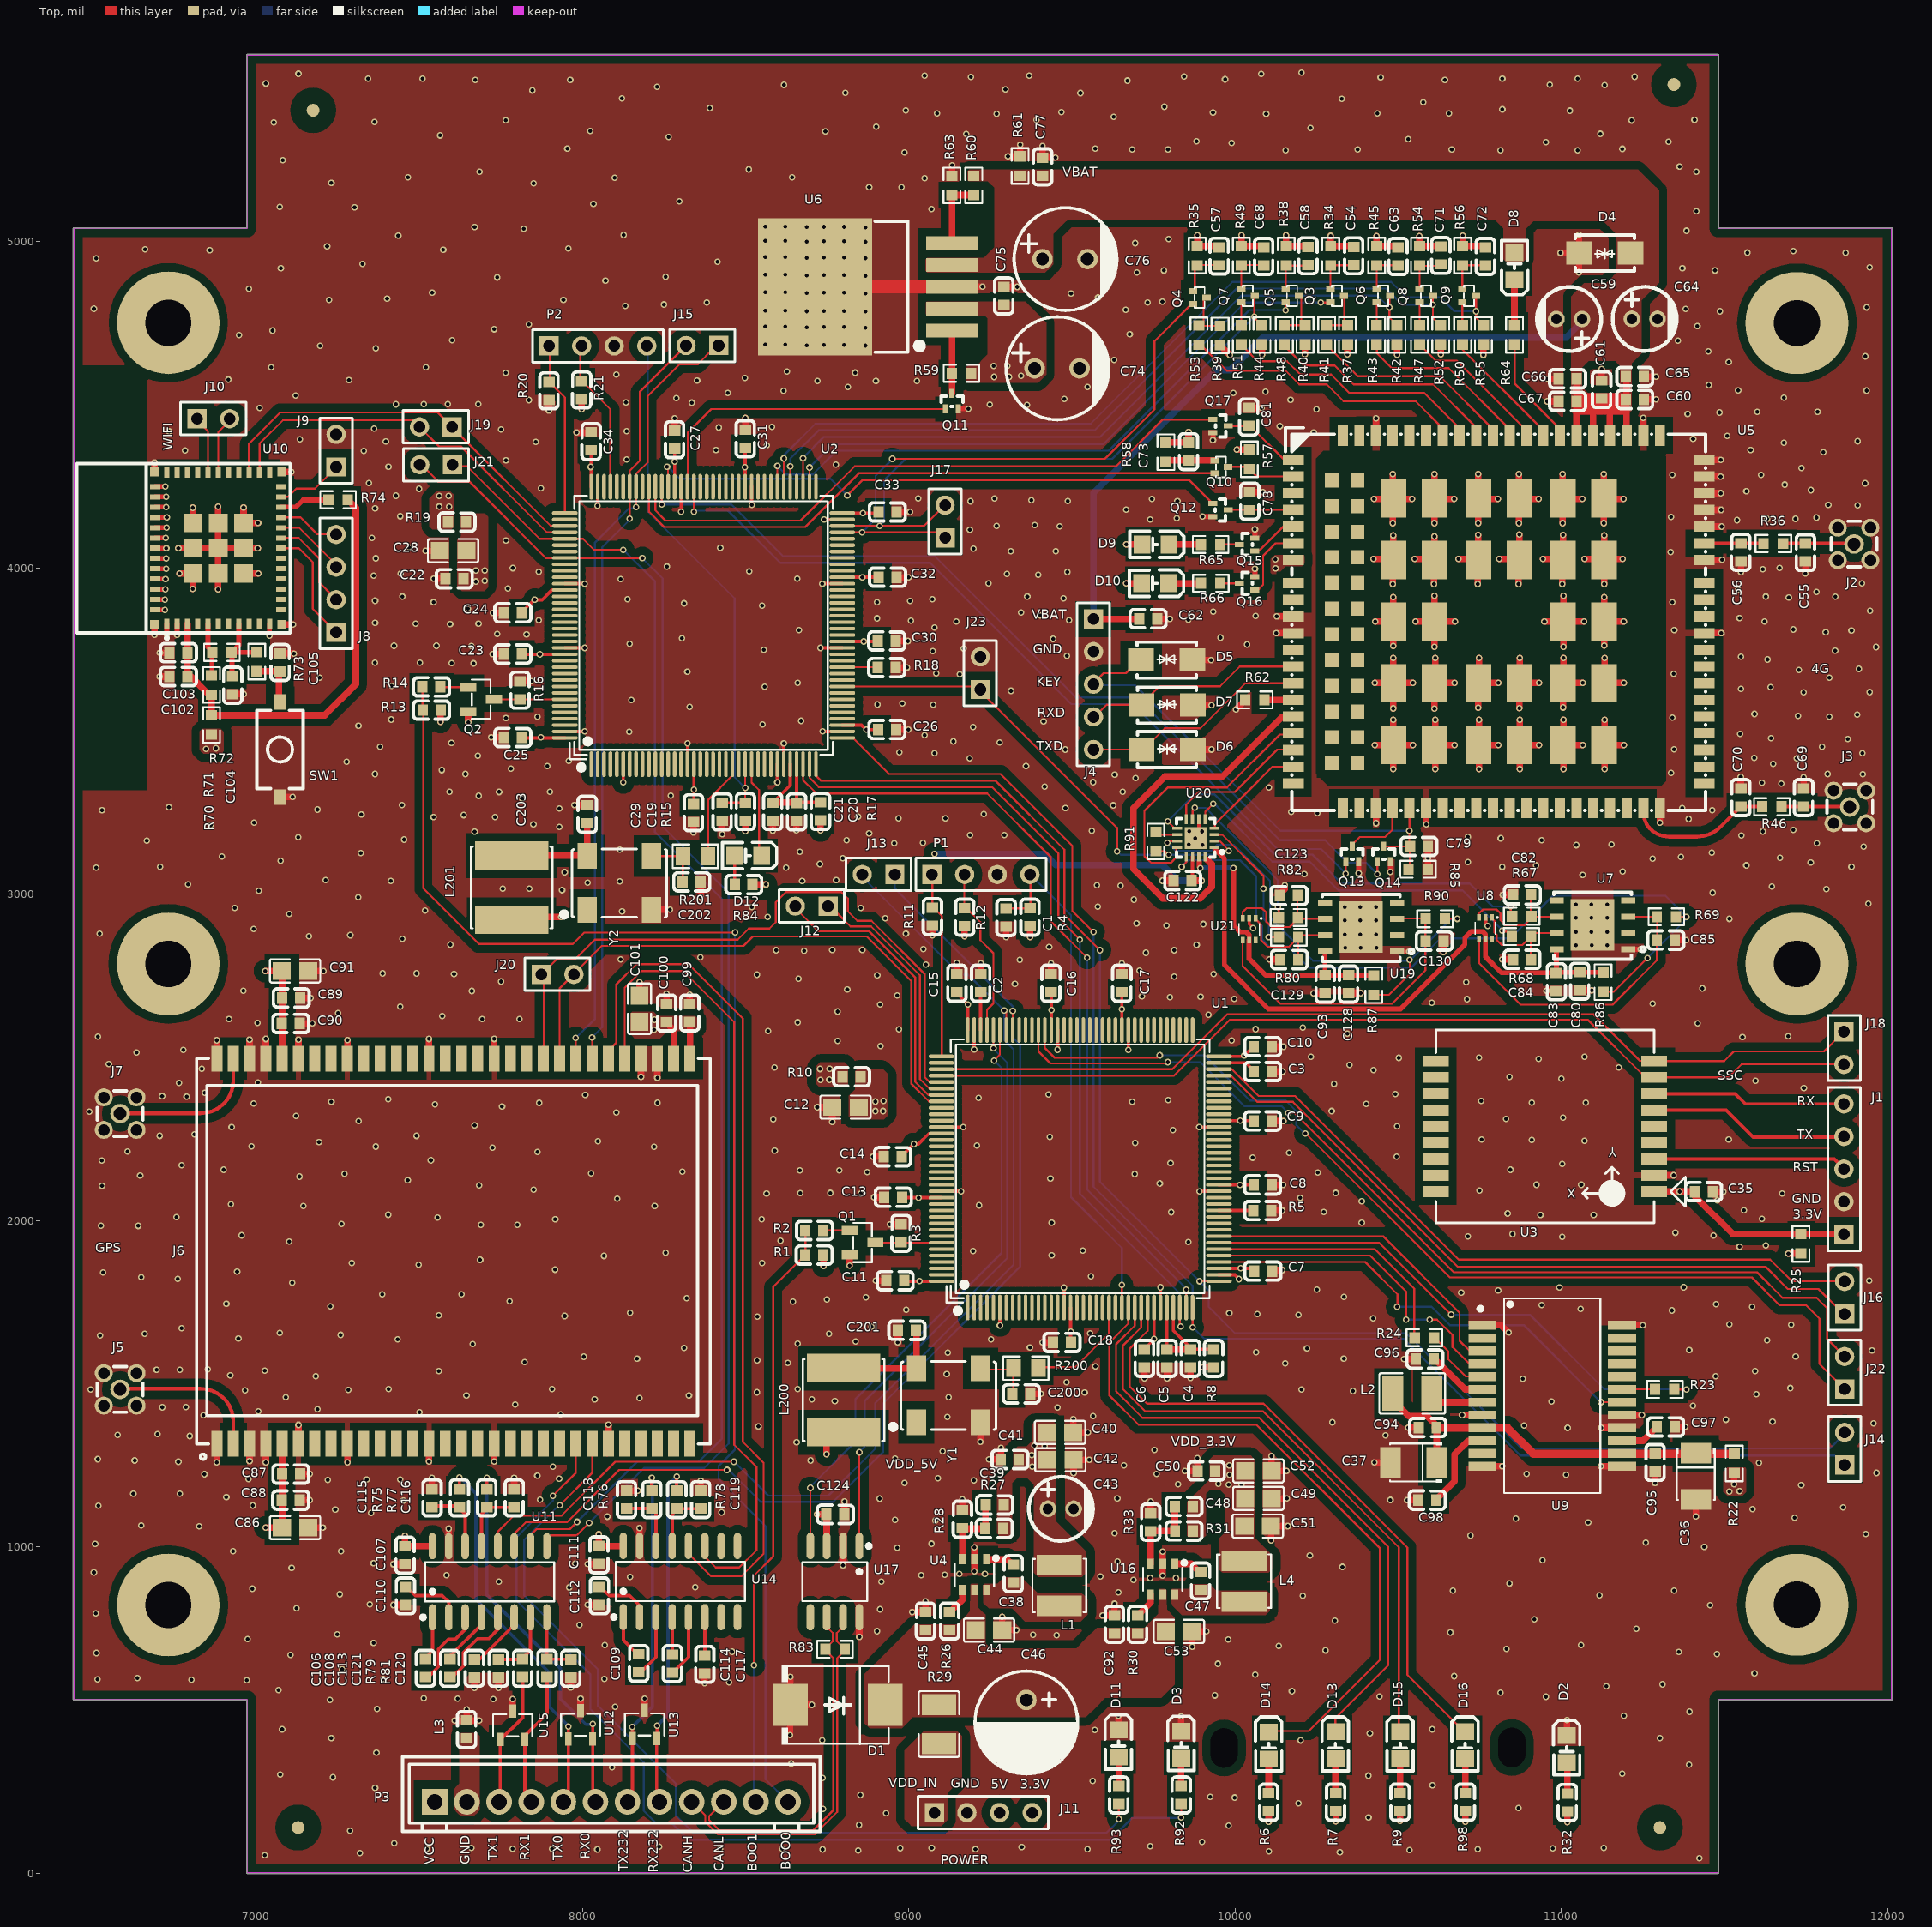
[diagram p0: Top view]
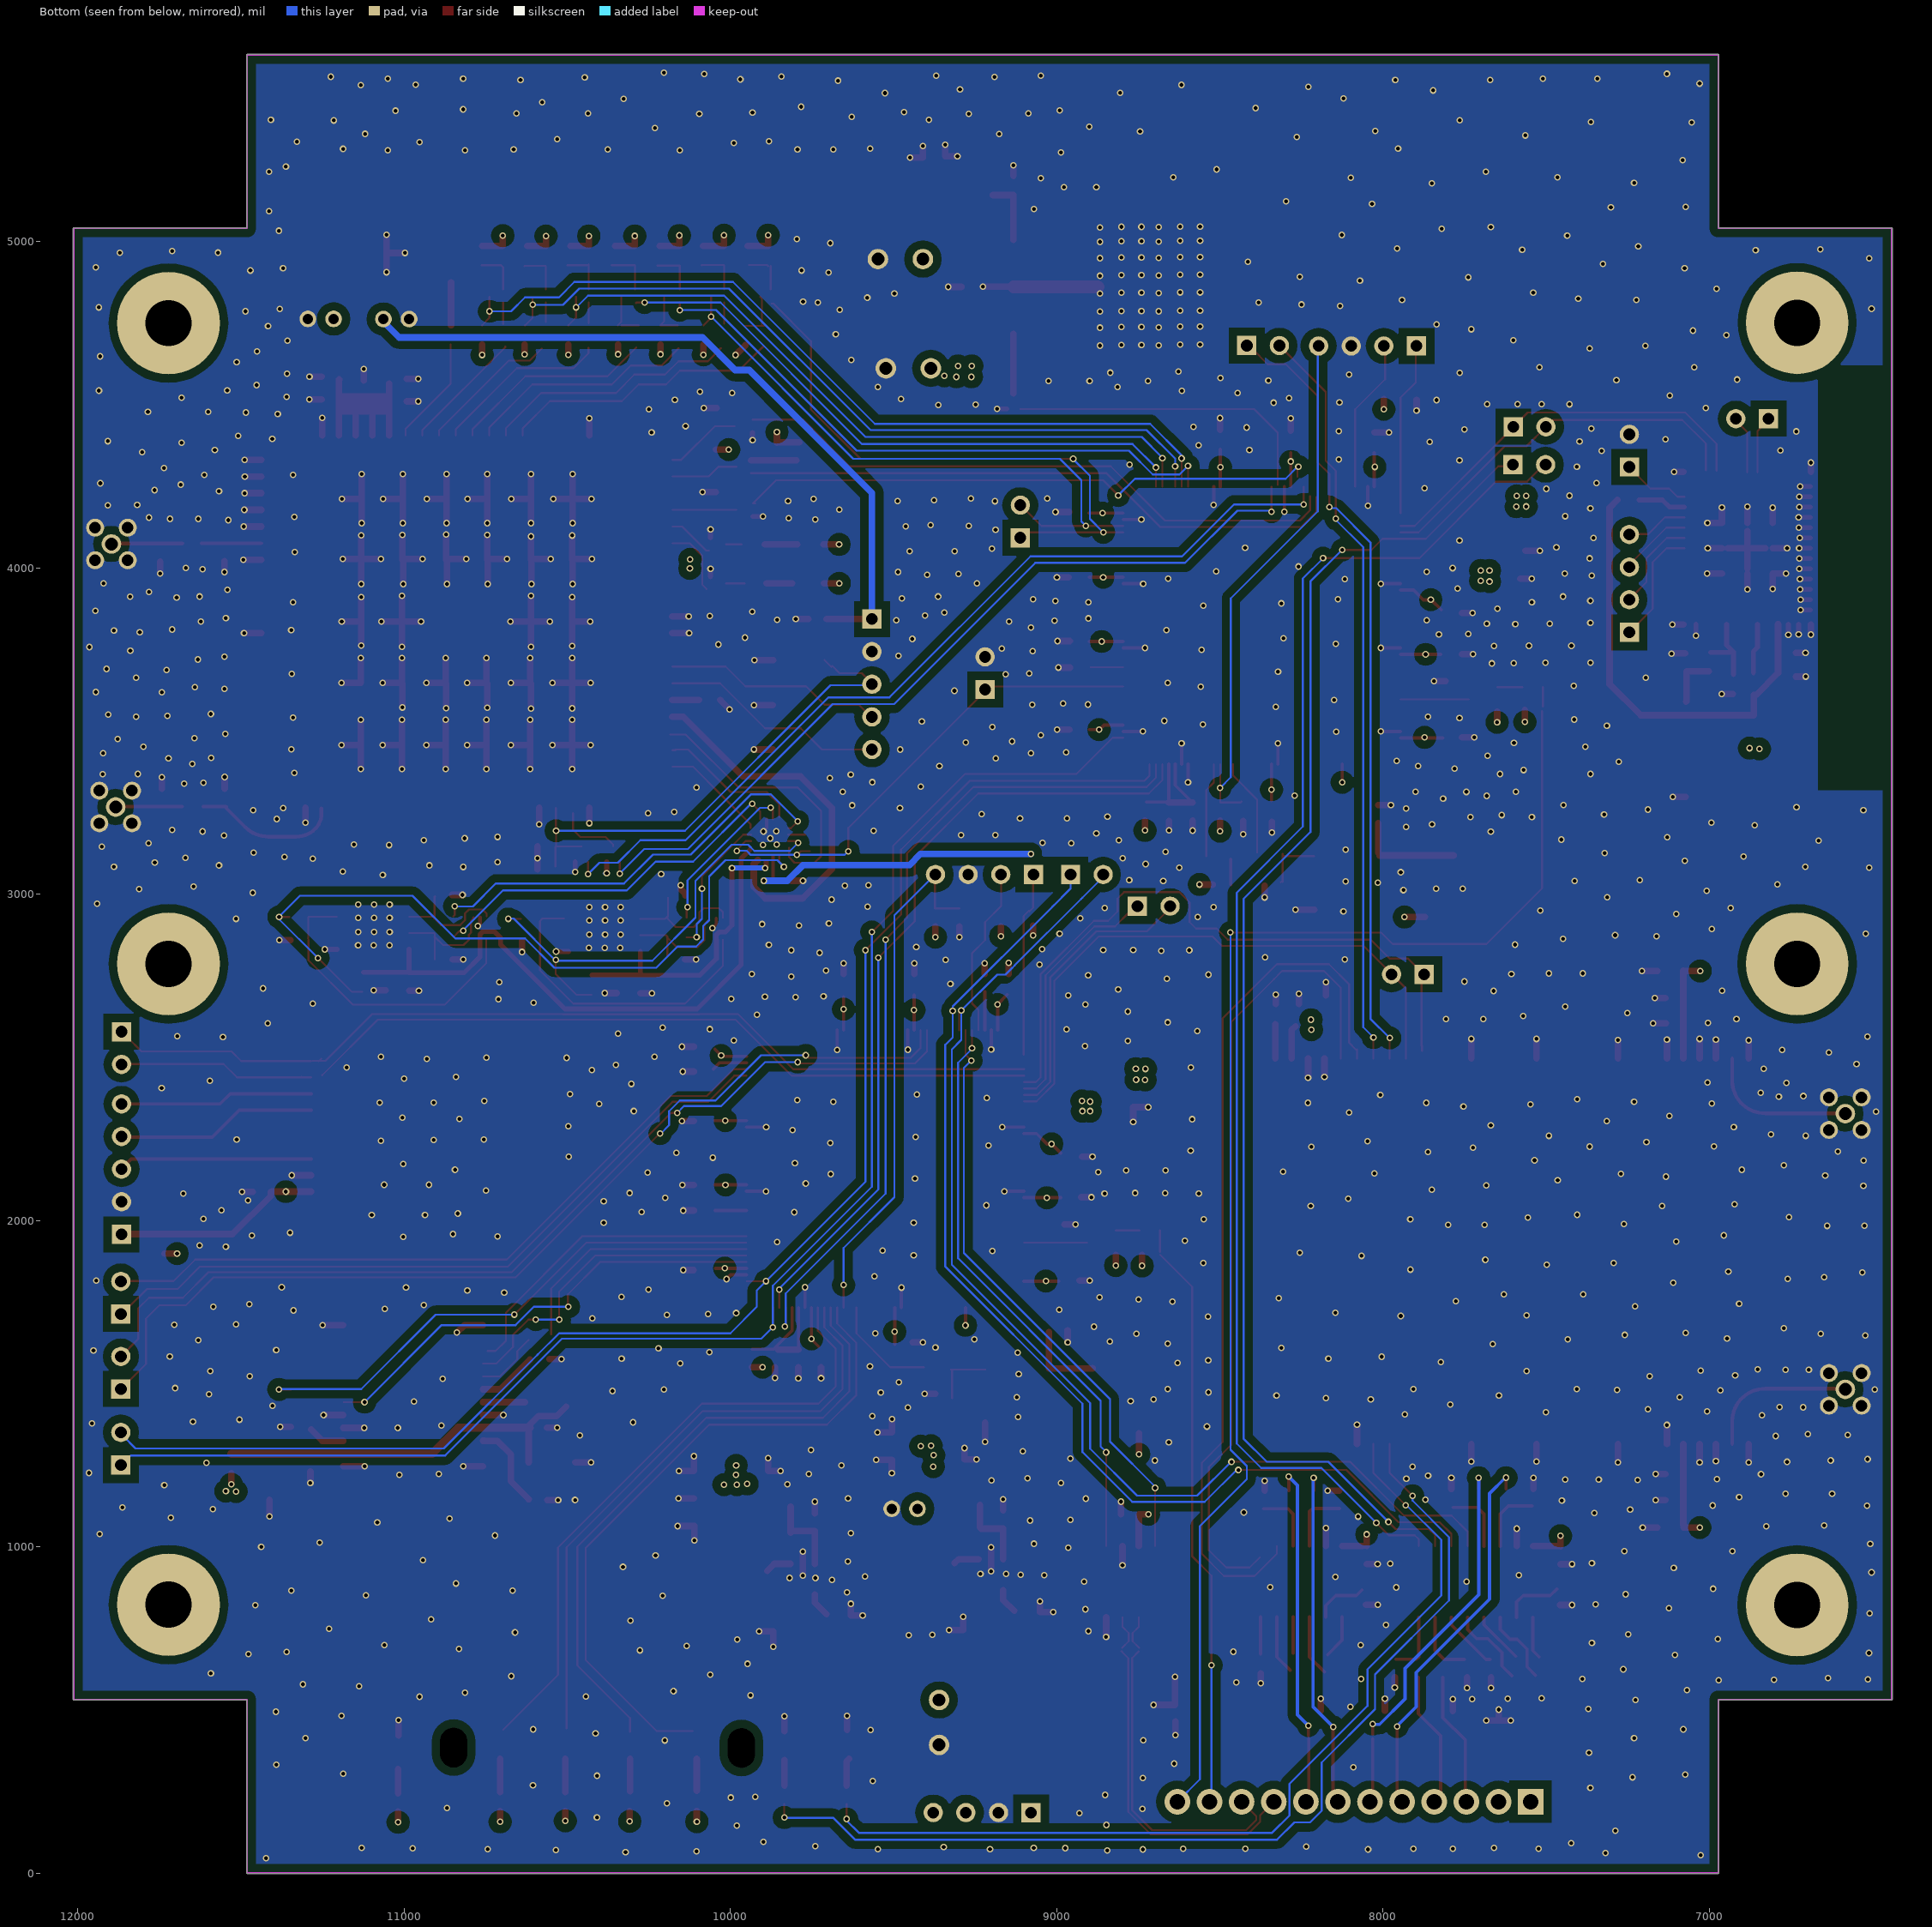
[diagram p1: Bottom view, seen from below]
# Altium PCB MISC86294.PcbDoc (part 1 of 8)
Units mil, origin at the board's own origin, x right, y up, seen from the top; angles counter-clockwise.
Board outline 5574.84 x 5574.84 mil, 4 copper layers (Top, GND02, PWR03, Bottom), stack 23.756 mil thick; 313 components, 311 nets, 1350 pads, 1701 vias.

## Layer stack, top to bottom
Top: signal copper 1.4
Dielectric: prepreg 2.8, PP-006, Dk 4.1
GND02: plane copper 1.378
Dielectric: dielectric 12.6, FR-4, Dk 4.8
PWR03: plane copper 1.378
Dielectric: prepreg 2.8, PP-006, Dk 4.1
Bottom: signal copper 1.4

## Board outline
6438.92,532.93 ccw(c6440.91,532.93) 6440.91,530.95 6970.42,530.95 6970.42,1.44 ccw(c6972.4,1.44) 6972.4,-0.55 11480.28,-0.55 ccw(c11480.28,1.44) 11482.26,1.44 11482.26,530.95 12011.78,530.95 ccw(c12011.78,532.93) 12013.76,532.93 12013.76,5040.81 ccw(c12011.78,5040.81) 12011.78,5042.79 11482.26,5042.79 11482.26,5572.31 ccw(c11480.28,5572.31) 11480.28,5574.29 6972.4,5574.29 ccw(c6972.4,5572.31) 6970.42,5572.31 6970.42,5042.79 6440.91,5042.79 ccw(c6440.91,5040.81) 6438.92,5040.81
cut-out: -1105,6605

## Design rules (kind name [scope] priority, off if disabled: settings)
Clearance Clearance_2 [HASPAD('free-MARK')] p1: gap=50
Clearance Clearance_1 [INPOLYGON] p2: gap=15
Clearance [All] p3: gap=6
DiffPairsRouting [All] p1: maxlimit=6 minlimit=6 mostfreqgap=6 maxuncoupledlength=500
PlaneClearance [All] p1: clearance=10
PlaneConnect [All] p1: planeconnectstyle=Direct reliefexpansion=20 reliefentries=4 reliefconductorwidth=10 reliefairgap=10
PolygonConnect [All] p1: connectstyle=Direct reliefconductorwidth=10 reliefentries=4 polygonreliefangle="90 Angle"
RoutingVias [All] p1: holewidth=12 width=20 viastyle="Through Hole" minholewidth=12 minwidth=20 maxholewidth=12 maxwidth=20
SilkscreenOverComponentPads SilkToSolderMaskClearance [IsPad] p1: minsilkscreentomaskgap=2
SolderMaskExpansion [All] p1: expansion=4
Width [All] p1: maxlimit=60 minlimit=6 preferedwidth=6 minimp=50.000000 maximp=50.000000 favimp=50.000000
24 further rules are at their usual default settings.

## Classes and differential pairs
component class "06 4G_Comm": C54 C55 C56 C57 C58 C59 C60 C61 C62 C63 C64 C65 C66 C67 C68 C69 C70 C71 C72 C73 C74 C75 C76 C77 C78 C79 C80 C81 C82 C83 C84 C85 C93 C122 C123 C128 C129 C130 D4 D5 D6 D7 D8 D9 D10 J2 J3 J4 J23 Q3 Q4 Q5 Q6 Q7 Q8 Q9 Q10 Q11 Q12 Q13 Q14 Q15 Q16 Q17 R34 R35 R36 R37 R38 R39 R40 R41 R42 R43 R44 R45 R46 R47 R48 R49 R50 R51 R52 R53 R54 R55 R56 R57 R58 R59 R60 R61 R62 R63 R64 R65 R66 R67 R68 R69 R80 R82 R85 R86 R87 R90 R91 U5 U6 U7 U8 U19 U20 U21
component class "09 Power": C38 C39 C40 C41 C42 C43 C44 C45 C46 C47 C48 C49 C50 C51 C52 C53 C92 D1 D2 J11 L1 L3 L4 R26 R27 R28 R29 R30 R31 R32 R33 U4 U16
component class "08 Interface": C106 C107 C108 C109 C110 C111 C112 C113 C114 C115 C116 C117 C118 C119 C120 C121 C124 J13 J14 J15 J16 J17 J18 J19 J20 J21 J22 P3 R75 R76 R77 R78 R79 R81 R83 U11 U12 U13 U14 U15 U17
component class "07 GPS_Gyro": C35 C36 C37 C86 C87 C88 C89 C90 C91 C94 C95 C96 C97 C98 C99 C100 C101 C102 C103 C104 C105 D3 D11 J1 J5 J6 J7 J8 J9 J10 L2 R22 R23 R24 R25 R70 R71 R72 R73 R74 R92 R93 SW1 U3 U9 U10
component class "04 MCU2": C19 C20 C21 C22 C23 C24 C25 C26 C27 C28 C29 C30 C31 C32 C33 C34 C202 C203 D12 L201 P2 Q2 R13 R14 R15 R16 R17 R18 R19 R20 R21 R84 R201 U2 Y2
component class "03 MCU1": C1 C2 C3 C4 C5 C6 C7 C8 C9 C10 C11 C12 C13 C14 C15 C16 C17 C18 C200 C201 D13 D14 D15 D16 J12 L200 P1 Q1 R1 R2 R3 R4 R5 R6 R7 R8 R9 R10 R11 R12 R98 R200 U1 Y1

## Components (designator, comment, footprint, x,y, rotation, side; value= is the part's Value field where it differs from the comment)
C1 "100nF/50V" 0603 9297.89,2929 r90 top
C2 "2.2uF/25V" C0603 9220,2727.62 r90 top
C3 "2.2uF/25V" C0603 10084,2457.11 r0 top
C4 "10uF/10V" C0603 9862.74,1578 r270 top
C5 "10uF/10V" C0603 9791.47,1578 r270 top
C6 "100nF/50V" C0603 9721.85,1578 r270 top
C7 "100nF/50V" C0603 10085,1845.7 r0 top
C8 "100nF/50V" C0603 10084,2109.55 r0 top
C9 "100nF/50V" C0603 10084,2305.4 r0 top
C10 "100nF/50V" C0603 10084,2533.26 r0 top
C11 "100nF/50V" C0603 8958,1815.89 r180 top
C12 "4.7uF/10V" C0805 8813,2348 r180 top
C13 "100nF/50V" C0603 8952.38,2071.72 r180 top
C14 "100nF/50V" C0603 8950.38,2195.95 r180 top
C15 "100nF/50V" C0603 9147.19,2727.62 r90 top
C16 "100nF/50V" C0603 9435.42,2727.62 r90 top
C17 "100nF/50V" C0603 9652.66,2727.62 r90 top
C18 "100nF/50V" C0603 9469.38,1626.89 r180 top
C19 "100nF/50V" 0603 8427.53,3253 r90 top
C20 "10uF/10V" C0603 8655.85,3253 r270 top
C21 "10uF/10V" C0603 8582.7,3254 r270 top
C22 "100nF/50V" C0603 7607,3967.45 r180 top
C23 "100nF/50V" C0603 7786,3736.6 r180 top
C24 "100nF/50V" C0603 7786,3862.74 r180 top
C25 "100nF/50V" C0603 7786,3480.89 r180 top
C26 "100nF/50V" C0603 8932.62,3505.51 r0 top
C27 "100nF/50V" C0603 8281.72,4393.62 r90 top
C28 "4.7uF/10V" C0805 7610.45,4053.47 r180 top
C29 "100nF/50V" C0603 8339.81,3250.38 r270 top
C30 "100nF/50V" C0603 8931.62,3776.58 r0 top
C31 "100nF/50V" C0603 8498.66,4396.62 r90 top
C32 "100nF/50V" C0603 8934.62,3972.11 r0 top
C33 "100nF/50V" C0603 8933.91,4172.12 r0 top
C34 "100nF/50V" C0603 8025.97,4388.06 r90 top
C35 "100nF/50V" 0603 11436,2089 r0 top
C36 "47uF/10V" CAP-SMD_L3.5-W2.8 11412,1216 r90 top
C37 "47uF/10V" CAP-SMD_L3.5-W2.8 10547,1259 r0 top
C38 "100nF/50V" 0603 9320,918 r90 top
C39 "100pF/50V" 0603 9263,1129 r180 top
C40 "22uF/10V" C0805 9456,1351 r0 top
C41 "100nF/50V" 0603 9310,1268 r180 top
C42 "22uF/10V" C0805 9457,1267 r0 top
C43 "100uF/10V" CAP-TH_BD5.0-P2.00-D0.8-FD 9466,1117 r0 top
C44 "10uF/25V" C0805 9253,745 r180 top
C45 "100nF/50V" 0603 9051,773 r270 top
C46 "470uF/25V" CAP-TH_BD8.0-P3.50-D1.0-FD 9360,461 r270 top
C47 "100nF/50V" 0603 9894,896 r90 top
C48 "100pF/50V" 0603 9843,1124 r180 top
C49 "22uF/10V" C0805 10064,1149 r0 top
C50 "100nF/50V" 0603 9912,1233 r180 top
C51 "22uF/10V" C0805 10062,1064 r0 top
C52 "22uF/10V" C0805 10064,1233 r0 top
C53 "10uF/25V" C0805 9835,741 r180 top
C54 "1nF/50V" C0603 10363.37,4957.2 r270 top
C55 "NM" C0603 11747.98,4047.68 r90 top
C56 "NM" C0603 11549.87,4048.68 r90 top
C57 "1nF/50V" C0603 9950.84,4956.2 r270 top
C58 "1nF/50V" C0603 10223.19,4957.2 r270 top
C59 "100uF/10V" RB5*7 11023.73,4763.25 r180 top
C60 "100nF/50V" C0603 11224.97,4516.75 r0 top
C61 "33pF/50V" C0603 11123.25,4546.97 r90 top
C62 "12pF/50V" C0603 9732.97,3844.75 r0 top
C63 "1nF/50V" C0603 10499.54,4955.2 r90 top
C64 "100uF/10V" RB5*7 11255.27,4763.84 r0 top
C65 "100nF/50V" C0603 11224.97,4586.84 r0 top
C66 "33pF/50V" C0603 11019.03,4580.16 r180 top
C67 "12pF/50V" C0603 11019.03,4510.93 r180 top
C68 "1nF/50V" C0603 10087.43,4955.2 r90 top
C69 "NM" C0603 11742.3,3296.93 r270 top
C70 "NM" C0603 11550,3297 r270 top
C71 "1nF/50V" C0603 10630.72,4958.2 r90 top
C72 "1nF/50V" C0603 10766.89,4955.2 r90 top
C73 "1nF/50V" C0603 9857.05,4357.07 r90 top
C74 "470uF/25V" RB8*11_5 9455,4612.33 r0 top
C75 "100nF/50V" C0603 9290.95,4834.15 r90 top
C76 "470uF/25V" RB8*11_5 9479.34,4947.02 r0 top
C77 "100nF/50V" C0603 9409.95,5230.1 r90 top
C78 "10nF" C0603 10044.84,4205.07 r90 top
C79 "10nF" C0603 10563.27,3147.03 r0 top
C80 "100nF/50V" C0603 11056,2734 r270 top
C81 "10nF" C0603 10041.39,4463.07 r90 top
C82 "33pF/50V" C0603 10880.33,2998.34 r180 top
C83 "33pF/50V" C0603 10984.55,2732.33 r270 top
C84 "33pF/50V" C0603 10879.33,2800.92 r180 top
C85 "33pF/50V" C0603 11320,2860 r0 top
C86 "10uF/25V" C0805 7126.05,1059.3 r180 top
C87 "100nF/50V" 0603 7105.69,1223.3 r0 top
C88 "100pF/50V" 0603 7105.39,1143.41 r0 top
C89 "100pF/50V" 0603 7106.99,2682.45 r180 top
C90 "100nF/50V" 0603 7105.62,2604.45 r180 top
C91 "10uF/25V" C0805 7125.88,2765.45 r180 top
C92 "100nF/50V" 0603 9630.11,763.07 r270 top
C93 "100nF/50V" C0603 10276,2725 r270 top
C94 "1uF/25V" 0603 10590.17,1365.87 r180 top
C95 "100nF/50V" 0603 11287.19,1259.01 r270 top
C96 "470nF/50V" 0603 10582,1576 r180 top
C97 "1uF/25V" 0603 11319.26,1367.81 r0 top
C98 "1uF/25V" 0603 10589,1143.39 r180 top
C99 "100pF/50V" 0603 8328.55,2636.74 r270 top
C100 "100nF/50V" 0603 8257.55,2636.5 r270 top
C101 "10uF/25V" C0805 8174.55,2656.88 r270 top
C102 "100nF/50V" C0603 6761.04,3667.57 r0 top
C103 "100nF/50V" C0603 6761.04,3740.57 r0 top
C104 "100nF/50V" C0603 6927.43,3641.04 r90 top
C105 "100nF/50V" C0603 7072.57,3710.96 r90 top
C106 "100nF/50V" 0603 7518.38,628.1 r90 top
C107 "100nF/50V" 0603 7456,975 r270 top
C108 "100nF/50V" 0603 7592.85,628.1 r90 top
C109 "100nF/50V" 0603 8171.88,643.1 r90 top
C110 "100nF/50V" 0603 7457.26,850.1 r270 top
C111 "100nF/50V" 0603 8050.01,975.8 r270 top
C112 "100nF/50V" 0603 8051.47,850.2 r270 top
C113 "100nF/50V" 0603 7668.04,628.1 r270 top
C114 "100nF/50V" 0603 8275.05,642.1 r90 top
C115 "15pF/50V" 0603 7538.75,1150.2 r270 top
C116 "15pF/50V" 0603 7790,1150.2 r270 top
C117 "100nF/50V" 0603 8374.64,640.1 r270 top
C118 "15pF/50V" 0603 8134.49,1145.2 r270 top
C119 "15pF/50V" 0603 8361.99,1145.2 r270 top
C120 "15pF/50V" 0603 7963.59,628.1 r270 top
C121 "15pF/50V" 0603 7741.93,628.1 r270 top
C122 "100nF/50V" C0603 9839,3042 r0 top
C123 "33pF/50V" C0603 10165.17,2996.13 r180 top
C124 "100nF/50V" C0603 8774.85,1100.07 r180 top
C128 "33pF/50V" C0603 10347.66,2725.33 r270 top
C129 "33pF/50V" C0603 10166.33,2800.45 r180 top
C130 "33pF/50V" C0603 10610.67,2857.08 r0 top
C200 "15pF/50V" C0603 9344.83,1469.05 r180 top
C201 "100nF/50V" C0603 8993.85,1664.05 r180 top
C202 "15pF/50V" C0603 8334.75,3038.18 r180 top
C203 "100nF/50V" C0603 8013.95,3245.83 r90 top
D1 "SMCJ18A" SMC_L6.9-W5.9-LS7.9-RD 8782,516 r0 top
D2 "RED" LED_0805 11016,385 r90 top
D3 "RED" LED_0805 9834,398 r90 top
D4 "SMAJ6.8CA" SMA 11132.95,4965.93 r0 top
D5 "SMAJ6.8CA" SMA 9790.05,3718.07 r180 top
D6 "SMAJ6.8CA" SMA 9791.05,3444.07 r180 top
D7 "SMAJ6.8CA" SMA 9791.05,3580.07 r180 top
D8 "GREEN" LED0805 10856.62,4920.75 r270 top
D9 "GREEN" LED0805 9760,4073 r0 top
D10 "GREEN" LED0805 9759,3954 r0 top
D11 "RED" LED_0805 9642,402 r90 top
D12 "RED" LED_0805 8512,3119 r0 top
D13 "RED" LED_0805 10306.97,396.49 r90 top
D14 "RED" LED_0805 10102.45,396.2 r90 top
D15 "RED" LED_0805 10505.41,396.49 r90 top
D16 "RED" LED_0805 10704.49,396.49 r90 top
J1 "HEADER 5" 2.54mm_paizhen_5pin 11866,2158 r180 top
J2 "MMCX-KE RF connector" MMCX-KE 11897,4074 r270 top
J3 "MMCX-KE RF connector" MMCX-KE 11883.95,3267.93 r0 top
J4 "HEADER 5" 2.54mm_paizhen_5pin 9565.93,3644.05 r0 top
J5 "MMCX-KE RF connector" MMCX-KE 6582.55,1482.99 r270 top
J6 "UM482/K823" UM482_K823 7604.01,1902.55 r90 top
J7 "MMCX-KE RF connector" MMCX-KE 6582.55,2328.01 r180 top
J8 "JTAG-4p-2.54-single-row pin header" HDR_1X4_254 7244.43,3953.04 r90 top
J9 "Boot Option-2.54-single-row pin header" HDR_1X2_254 7244.43,4360.04 r90 top
J10 "Boot Option-2.54-single-row pin header" HDR_1X2_254 6868,4458 r0 top
J11 "Single-row straight pin header" HDR1X4 9078,186 r0 top
J12 "Boot Option-2.54-single-row pin header" HDR_1X2_254 8702,2964 r180 top
J13 "Boot Option-2.54-single-row pin header" HDR_1X2_254 8907,3061 r180 top
J14 "Boot Option-2.54-single-row pin header" HDR_1X2_254 11868,1301 r90 top
J15 "Boot Option-2.54-single-row pin header" HDR_1X2_254 8367,4682 r180 top
J16 "Boot Option-2.54-single-row pin header" HDR_1X2_254 11868,1764 r90 top
J17 "Boot Option-2.54-single-row pin header" HDR_1X2_254 9111,4143 r90 top
J18 "Boot Option-2.54-single-row pin header" HDR_1X2_254 11866,2529 r270 top
J19 "Boot Option-2.54-single-row pin header" HDR_1X2_254 7550,4433 r180 top
J20 "Boot Option-2.54-single-row pin header" HDR_1X2_254 7923,2755 r0 top
J21 "Boot Option-2.54-single-row pin header" HDR_1X2_254 7551,4317 r180 top
J22 "Boot Option-2.54-single-row pin header" HDR_1X2_254 11868,1534 r90 top
J23 "Boot Option-2.54-single-row pin header" HDR_1X2_254 9219,3678 r90 top
L1 "2.2uH/2A" IND-SMD_L4.0-W4.0 9461,882 r90 top
L2 "47uH±20%" 1210 10430.07,1475.15 r0 top locked
L3 "120Ω ±25% @100MHz" 0603 7644.48,440.39 r90 top
L4 "2.2uH/2A" IND-SMD_L4.0-W4.0 10027.31,895.03 r90 top
L200 "1uH 10%" SMD_L6.0-W6.0 8799.83,1450.05 r270 top
L201 "1uH 10%" SMD_L6.0-W6.0 7782.37,3020.86 r270 top
P1 "Single-row straight pin header" HDR1X4 9071,3061 r0 top
P2 "Single-row straight pin header" HDR1X4 7896.84,4680.88 r0 top
P3 "Through-hole pad, 2mm pitch" XH-12A 8088.37,219.05 r0 top
Q1 "8550" SOT-23-SS8550 8858,1933 r180 top
Q2 "8550" SOT-23-SS8550 7688.81,3597.92 r180 top
Q3 "2SC4617TLQ" EMT3 10312.73,4834.14 r180 top
Q4 "2SC4617TLQ" EMT3 9891.8,4829.14 r180 top
Q5 "2SC4617TLQ" EMT3 10175.45,4834.14 r180 top
Q6 "2SC4617TLQ" EMT3 10454.9,4834.14 r180 top
Q7 "2SC4617TLQ" EMT3 10039.29,4834.14 r180 top
Q8 "2SC4617TLQ" EMT3 10586.08,4834.14 r180 top
Q9 "2SC4617TLQ" EMT3 10717.25,4834.14 r180 top
Q10 "2SC4617TLQ" EMT3 9957.49,4310.29 r180 top
Q11 "DTC043ZEBTL" SOT-416_L1_6-W0_8-P1_00-LS1_6-BR 9132.04,4509.85 r270 top
Q12 "DTC043ZEBTL" SOT-416_L1_6-W0_8-P1_00-LS1_6-BR 9953.08,4178.05 r180 top
Q13 "DTC043ZEBTL" SOT-416_L1_6-W0_8-P1_00-LS1_6-BR 10358.93,3121.89 r270 top
Q14 "DTC043ZEBTL" SOT-416_L1_6-W0_8-P1_00-LS1_6-BR 10455.68,3121.89 r270 top
Q15 "DTC043ZEBTL" SOT-416_L1_6-W0_8-P1_00-LS1_6-BR 10038.59,4072.48 r0 top
Q16 "DTC043ZEBTL" SOT-416_L1_6-W0_8-P1_00-LS1_6-BR 10038.59,3953.48 r0 top
Q17 "DTC043ZEBTL" SOT-416_L1_6-W0_8-P1_00-LS1_6-BR 9954.08,4435.6 r180 top
R1 "10K" 0603 8709.75,1895 r0 top
R2 "10K" 0603 8710.75,1969.89 r180 top
R3 "10K" 0603 8976,1961.25 r270 top
R4 "10K" 0603 9371.16,2930 r270 top
R5 "10K" 0603 10084,2031 r180 top
R6 "NA" 0603 10102.7,217.71 r90 top
R7 "NA" 0603 10307.97,217.71 r90 top
R8 "120R@100MHz" 0603 9934,1578 r90 top
R9 "NA" 0603 10505.41,217.71 r90 top
R10 "0R" 0603 8824,2441 r0 top
R11 "10K" 0603 9072,2931.78 r270 top
R12 "10K" 0603 9171,2930 r270 top
R13 "10K" 0603 7536.75,3565 r0 top
R14 "10K" 0603 7537,3635.84 r180 top